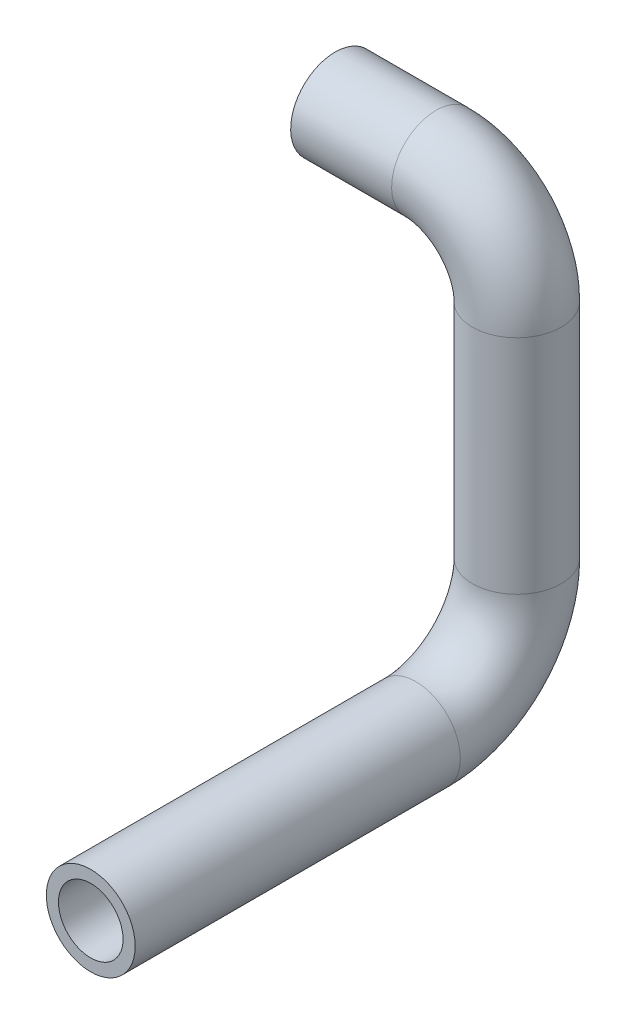
SolidWorks part; units mm, degrees
ref_plane "Front Plane" through (0, 0, 0) normal (0, 0, 1) x (1, 0, 0)
ref_plane "Top Plane" through (0, 0, 0) normal (0, 1, 0) x (1, 0, 0)
ref_plane "Right Plane" through (0, 0, 0) normal (1, 0, 0) x (0, 0, -1)
sketch "Sketch 1" plane through (0, 0, 0) normal (0, 0, 1) x (1, 0, 0)
  line L0 (0, 0) -> (25, 0)
  line L1 (45, -20) -> (45, -50)
  arc A0 (25, 0) -> (45, -20) centre (25, -20) cw
  point P6 (45, 0)
  dimension "D2" = 20
  dimension "D1" = 45
  dimension "D3" = 50
sketch "Sketch 2" plane through (0, 0, 0) normal (1, 0, 0) x (0, 0, -1)
  circle A0 centre (0, 0) radius 11
  circle A1 centre (0, 0) radius 8
  dimension "D1" = 22
  dimension "D2" = 3
sweep "Sweep 1" add profiles "Sketch 2" path "Sketch 1"
ref_plane "Plane 1" through (45, 0, 0) normal (1, 0, 0) x (0, 0, -1)
sketch "Sketch 3" plane through (45, 0, 0) normal (1, 0, 0) x (0, 0, -1)
  line L0 (0, -50) -> (0, -75)
  line L1 (-11, -50) -> (11, -50) construction
  line L2 (-25, -100) -> (-105.5, -100)
  arc A0 (0, -75) -> (-25, -100) centre (-25, -75) cw
  point P8 (0, -100)
  dimension "D2" = 25
  dimension "D1" = 105.5
  dimension "D3" = 50
sketch "Sketch 4" plane through (0, -50, 0) normal (0, -1, 0) x (1, 0, 0)
  circle A0 centre (45, 0) radius 8 construction
  circle A1 centre (45, 0) radius 11
  circle A2 centre (45, 0) radius 11
  circle A3 centre (45, 0) radius 8
  dimension "D1" = 0
sweep "Sweep 2" add profiles "Sketch 4" path "Sketch 3"
